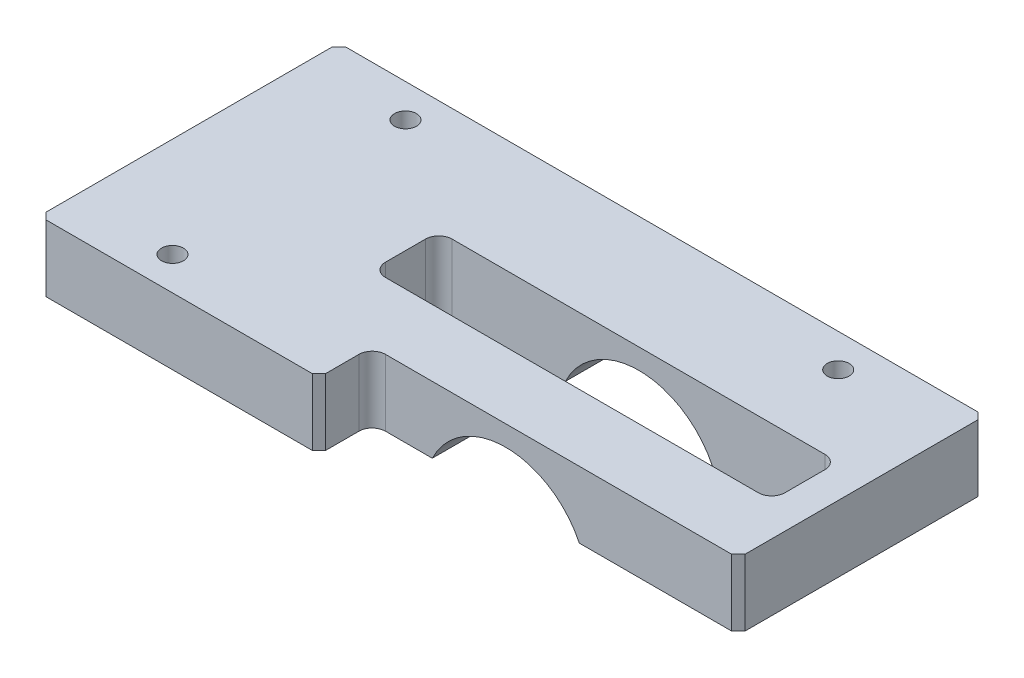
SolidWorks part; units mm, degrees
ref_plane "Front Plane" through (0, 0, 0) normal (0, 0, 1) x (1, 0, 0)
ref_plane "Top Plane" through (0, 0, 0) normal (0, 1, 0) x (1, 0, 0)
ref_plane "Right Plane" through (0, 0, 0) normal (1, 0, 0) x (0, 0, -1)
sketch "Sketch1" plane through (0, 0, 0) normal (0, 1, 0) x (1, 0, 0)
  line L1 (-145, 22.5) -> (145, 22.5)
  line L2 (-145, 22.5) -> (-145, -22.5)
  line L3 (-145, -22.5) -> (145, -22.5)
  line L4 (145, 22.5) -> (145, -22.5)
  line L5 (-145, 22.5) -> (145, -22.5) construction
  line L6 (-145, -22.5) -> (145, 22.5) construction
  point P0 (0, 0)
  dimension "D1" = 290
  dimension "D2" = 45
extrude "Boss-Extrude1" add sketch "Sketch1" along normal blind 10
sketch "Sketch3" plane through (0, 10, 0) normal (0, 1, 0) x (1, 0, 0)
  line L0 (-145, 22.5) -> (-145, -22.5) construction
  line L2 (-145, 0.5) -> (49855, 0.5) construction
  line L4 (-145, -22.5) -> (145, -22.5) construction
  line L8 (-135, 5.5) -> (-75, 5.5)
  line L9 (-135, 5.5) -> (-135, -4.5)
  line L10 (-135, -4.5) -> (-75, -4.5)
  line L11 (-75, 5.5) -> (-75, -4.5)
  line L12 (-135, 5.5) -> (-75, -4.5) construction
  line L13 (-135, -4.5) -> (-75, 5.5) construction
  point P10 (-105, 0.5)
  dimension "D1" = 23
  dimension "D2" = 10
  dimension "D3" = 10
extrude "Cut-Extrude2" cut sketch "Sketch3" against normal blind 10
sketch "Sketch4" plane through (-145, 0, 0) normal (-1, 0, 0) x (0, 0, 1)
  line L1 (-22.5, 10) -> (22.5, 10)
  line L2 (-22.5, 10) -> (-22.5, 0)
  line L3 (-22.5, 0) -> (22.5, 0)
  line L4 (22.5, 10) -> (22.5, 0)
extrude "Boss-Extrude2" add sketch "Sketch4" along normal blind 22
sketch "Sketch6" plane through (0, 10, 0) normal (0, 1, 0) x (1, 0, 0)
  line L1 (-167, -22.5) -> (145, -22.5) construction
  line L2 (-167, -22.5) -> (-167, 22.5) construction
  circle A0 centre (-10, 0.5) radius 5
  circle A1 centre (-50, 0.5) radius 5
  dimension "D2" = 40
  dimension "D4" = 10
  dimension "D1" = 117
  dimension "D3" = 23
extrude "Cut-Extrude4" cut sketch "Sketch6" against normal blind 30
sketch "Sketch7" plane through (0, 0, 0) normal (0, -1, 0) x (1, 0, 0)
  line L0 (10, -0.5) -> (-49990, -0.5) construction
  line L1 (-30, 2) -> (-30, -49998) construction
  line L3 (-70, 12) -> (10, 12)
  line L4 (-70, 12) -> (-70, -13)
  line L5 (-70, -13) -> (10, -13)
  line L6 (10, 12) -> (10, -13)
  line L7 (-70, 12) -> (10, -13) construction
  line L8 (-70, -13) -> (10, 12) construction
  line L10 (-167, 22.5) -> (145, 22.5) construction
  circle A0 centre (-50, -0.5) radius 5 construction
  circle A1 centre (-10, -0.5) radius 5 construction
  point P10 (-30, -0.5)
  point P15 (10, -0.5)
  dimension "D1" = 25
  dimension "D2" = 80
  dimension "D3" = 23
extrude "Cut-Extrude5" cut sketch "Sketch7" against normal blind 27
sketch "Sketch9" plane through (0, 10, 0) normal (0, 1, 0) x (1, 0, 0)
  line L0 (145, 22.5) -> (-167, 22.5) construction
  line L1 (-70, 22.5) -> (10, 22.5)
  line L2 (-70, 22.5) -> (-70, -22.5)
  line L3 (-70, -22.5) -> (10, -22.5)
  line L4 (10, 22.5) -> (10, -22.5)
  line L5 (-167, -22.5) -> (145, -22.5) construction
  line L6 (-70, 13) -> (-70, -12) construction
  line L7 (10, -12) -> (10, 13) construction
extrude "Cut-Extrude7" cut sketch "Sketch9" against normal blind 42
sketch "Sketch10" plane through (0, 0, 22.5) normal (0, 0, 1) x (1, 0, 0)
  line L0 (145, 0) -> (145, 5)
  line L1 (145, 10) -> (145, 0) construction
  line L2 (145, 5) -> (130, 0)
  line L3 (10, 0) -> (145, 0) construction
  line L4 (130, 0) -> (145, 0)
  dimension "D1" = 5
  dimension "D2" = 15
extrude "Cut-Extrude8" cut sketch "Sketch10" against normal blind 20
sketch "Sketch13" plane through (0, 0, 22.5) normal (0, 0, 1) x (1, 0, 0)
  line L1 (-70, 10) -> (153.2108, 10)
  line L2 (-70, 10) -> (-70, 0)
  line L3 (-70, 0) -> (153.2108, 0)
  line L4 (153.2108, 10) -> (153.2108, 0)
extrude "Cut-Extrude11" cut sketch "Sketch13" against normal blind 105
hole_wizard "M5 Tapped Hole1" positions "3DSketch1" profile "Sketch15" tap size "M5" standard "Gb"
sketch3d "3DSketch1"
  line L1 (-70, 0, -22.5) -> (-70, 10, -22.5) construction
  line L2 (-70, 10, -22.5) -> (-167, 10, -22.5) construction
  point P0 (-159, 5, -22.5)
  point P2 (-81, 5, -22.5)
  dimension "D1" = 11
  dimension "D2" = 78
  dimension "D3" = 5
sketch "Sketch15" plane through (-159, 5, -22.5) normal (1, 0, 0) x (0, 1, 0)
  line L0 (0, 0) -> (0, 13.6618)
  line L1 (0, 13.6618) -> (2.1, 12.4)
  line L2 (2.1, 12.4) -> (2.1, 0)
  line L5 (2.1, 0) -> (0, 0)
  line L10 (0, 13.6618) -> (-2.1, 12.4) construction
  line L11 (0, -6.35) -> (0, 107.95) construction
  dimension "螺纹孔钻头直径" = 4.2
  dimension "螺纹孔钻头深度" = 12.4
  dimension "导头角度" = 118
cosmetic thread "Cosmetic Thread1" parameters "D1"=10, "D2"=5
cosmetic thread "Cosmetic Thread2" parameters "D1"=10, "D2"=5
sketch "Sketch19" plane through (0, 10, 0) normal (0, 1, 0) x (1, 0, 0)
  line L1 (-70, -22.5) -> (-125, -22.5)
  line L2 (-70, -22.5) -> (-70, -14.5)
  line L3 (-70, -14.5) -> (-125, -14.5)
  line L4 (-125, -22.5) -> (-125, -14.5)
  dimension "D1" = 55
  dimension "D2" = 8
extrude "Cut-Extrude13" cut sketch "Sketch19" against normal through all
sketch "Sketch20" plane through (0, 0, 22.5) normal (0, 0, 1) x (1, 0, 0)
  line L0 (-104.93, 10) -> (-104.93, -49990) construction
  line L1 (-70, 10) -> (-125, 10) construction
  line L2 (-167, 10) -> (-167, 0) construction
  line L3 (-70, 0) -> (-125, 0) construction
  line L4 (-117.93, 0) -> (-91.93, 0) construction
  line L5 (-117.93, 0) -> (-117.93, 7) construction
  line L6 (-117.93, 7) -> (-91.93, 7) construction
  line L7 (-91.93, 0) -> (-91.93, 7) construction
  circle A0 centre (-104.93, -5.3) radius 12.25
  point P5 (-167, 5)
  dimension "D4" = 24.5
  dimension "D5" = 15.3
  dimension "D1" = 62.07
  dimension "D2" = 26
  dimension "D3" = 7
extrude "Cut-Extrude14" cut sketch "Sketch20" against normal through all
hole_wizard "M4 Tapped Hole1" positions "3DSketch2" profile "Sketch24" tap size "M4" standard "Gb"
sketch3d "3DSketch2"
  line L0 (-167, 10, 22.5) -> (-167, 10, -22.5) construction
  line L1 (-70, 10, -22.5) -> (-167, 10, -22.5) construction
  line L2 (-167, 10, 22.5) -> (-125, 10, 22.5) construction
  point P0 (-152, 10, -17.5)
  point P7 (-87, 10, -17.5)
  point P9 (-152, 10, 17.5)
  dimension "D1" = 15
  dimension "D2" = 5
  dimension "D3" = 65
  dimension "D4" = 5
sketch "Sketch24" plane through (-152, 10, -17.5) normal (1, 0, 0) x (0, 0, 1)
  line L0 (0, 0) -> (0, 11.0914)
  line L1 (0, 11.0914) -> (1.65, 10.1)
  line L2 (1.65, 10.1) -> (1.65, 0)
  line L5 (1.65, 0) -> (0, 0)
  line L10 (0, 11.0914) -> (-1.65, 10.1) construction
  line L11 (0, -6.35) -> (0, 107.95) construction
  dimension "螺纹孔钻头直径" = 3.3
  dimension "螺纹孔钻头深度" = 10.1
  dimension "导头角度" = 118
cosmetic thread "Cosmetic Thread3" parameters "D1"=8, "D2"=4
cosmetic thread "Cosmetic Thread4" parameters "D1"=8, "D2"=4
cosmetic thread "Cosmetic Thread5" parameters "D1"=8, "D2"=4
chamfer "Chamfer1" distance 1 angle 45 5 edges at (-70, 5, -22.5) (-70, 5, 14.5) (-167, 5, -22.5) (-167, 5, 22.5) (-125, 5, 22.5)
fillet "Fillet1" radius 2 1 edges at (-125, 5, 14.5)
fillet "Fillet2" radius 2 4 edges at (-75, 5, -5.5) (-75, 5, 4.5) (-135, 5, -5.5) (-135, 5, 4.5)
